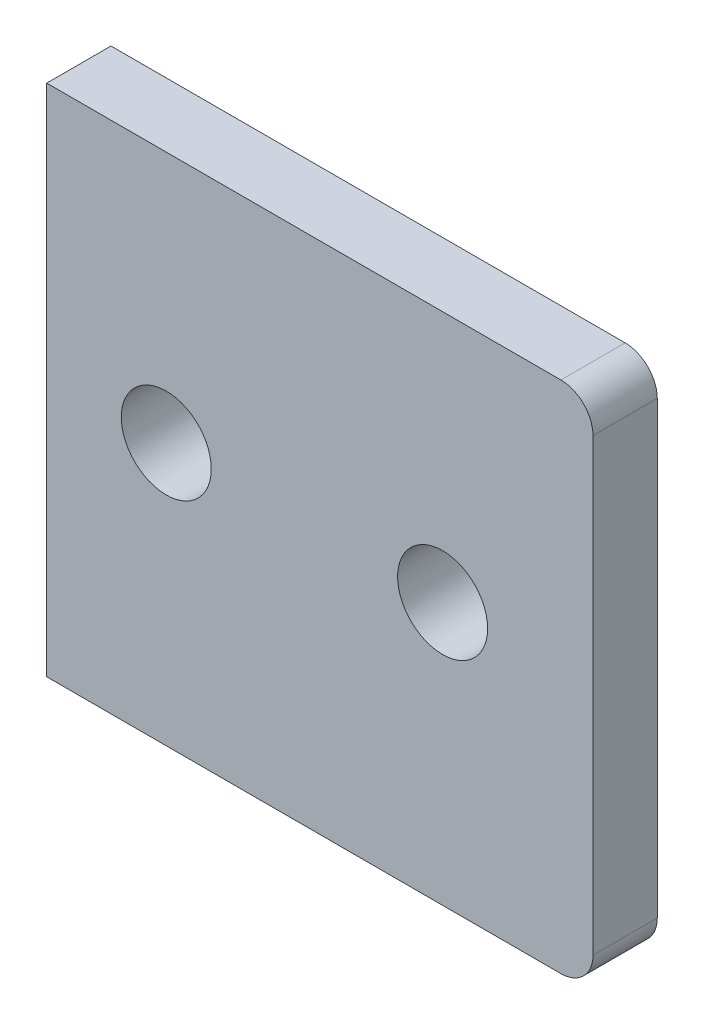
from build123d import *

# Parameters (mm, degrees)
EXTRUDE_1_DEPTH             = 10
HOLE_WIZARD_14_0_14_1_D     = 14
HOLE_WIZARD_14_0_14_1_DEPTH = 19.793975667
HOLE_WIZARD_14_0_14_1_TIP   = 4.206024333


with BuildPart() as part:
    # 草图1 → 凸台-拉伸1 (new body)
    with BuildSketch(Plane.XY):
        with BuildLine():
            Line((-42.5, 40), (37.5, 40))
            ThreePointArc((37.5, 40), (41.035533906, 38.535533906), (42.5, 35))
            Line((42.5, 35), (42.5, -35))
            ThreePointArc((42.5, -35), (41.035533906, -38.535533906), (37.5, -40))
            Line((37.5, -40), (-42.5, -40))
            Line((-42.5, -40), (-42.5, 40))
        make_face()
    extrude(amount=EXTRUDE_1_DEPTH)

    # Ø14.0 (14) 直径孔1
    with Locations(Plane.XY.offset(10)):
        with Locations((19.1, 0.8), (-23.9, 0.8)):
            Hole(HOLE_WIZARD_14_0_14_1_D / 2, depth=HOLE_WIZARD_14_0_14_1_DEPTH)
            with Locations((0, 0, -(HOLE_WIZARD_14_0_14_1_DEPTH + HOLE_WIZARD_14_0_14_1_TIP / 2))):  # 118° drill point
                Cone(0, HOLE_WIZARD_14_0_14_1_D / 2, HOLE_WIZARD_14_0_14_1_TIP, mode=Mode.SUBTRACT)


solid = part.part
